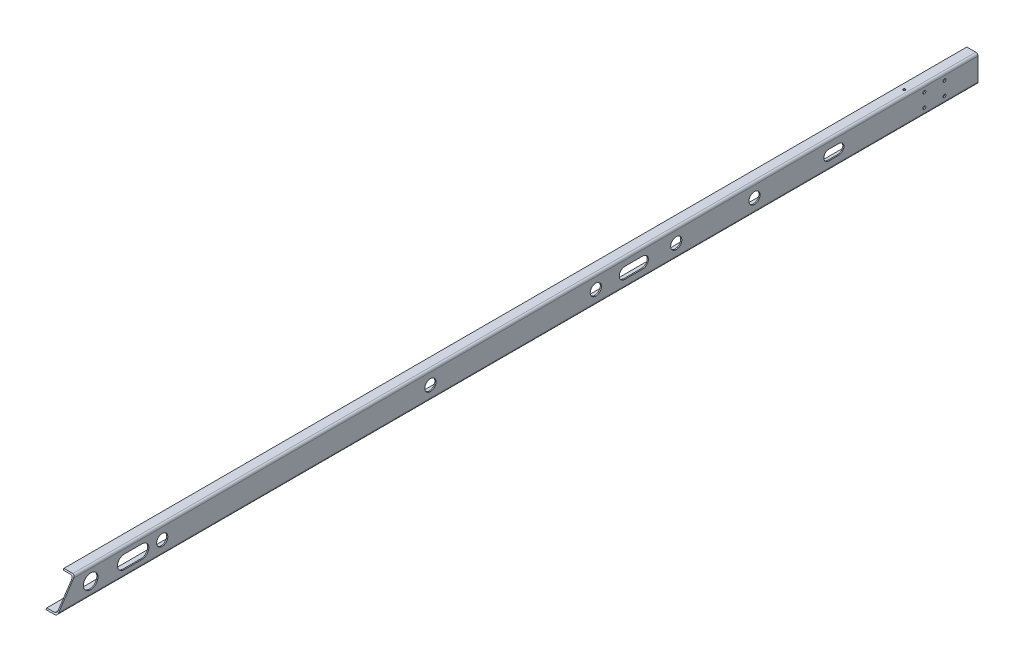
SolidWorks part; units mm, degrees
ref_plane "前视基准面" through (0, 0, 0) normal (0, 0, 1) x (1, 0, 0)
ref_plane "上视基准面" through (0, 0, 0) normal (0, 1, 0) x (1, 0, 0)
ref_plane "右视基准面" through (0, 0, 0) normal (1, 0, 0) x (0, 0, -1)
sketch "草图1" plane through (0, 0, 0) normal (0, 0, 1) x (1, 0, 0)
  line L24 (626.1756, -48.4289) -> (666.1756, -48.4289)
  line L25 (676.1756, -38.4289) -> (676.1756, 61.5711)
  line L26 (666.1756, 71.5711) -> (626.1756, 71.5711)
  line L27 (626.1756, 71.5711) -> (626.1756, 66.5711)
  line L28 (626.1756, 66.5711) -> (661.1756, 66.5711)
  line L29 (671.1756, 56.5711) -> (671.1756, -33.4289)
  line L30 (661.1756, -43.4289) -> (626.1756, -43.4289)
  line L31 (626.1756, -43.4289) -> (626.1756, -48.4289)
  arc A12 (666.1756, -48.4289) -> (676.1756, -38.4289) centre (666.1756, -38.4289) ccw
  arc A13 (676.1756, 61.5711) -> (666.1756, 71.5711) centre (666.1756, 61.5711) ccw
  arc A14 (671.1756, 56.5711) -> (661.1756, 66.5711) centre (661.1756, 56.5711) ccw
  arc A15 (661.1756, -43.4289) -> (671.1756, -33.4289) centre (661.1756, -33.4289) ccw
extrude "凸台-拉伸1" add sketch "草图1" along normal blind 4120
sketch "草图2" plane through (0, 71.5711, 0) normal (0, 1, 0) x (1, 0, 0)
  line L0 (626.1756, 0) -> (676.1756, 0)
  line L1 (651.1756, 0) -> (651.1756, -305)
  circle A0 centre (651.1756, -305) radius 5
extrude "切除-拉伸1" cut sketch "草图2" against normal blind 10
sketch "草图3" plane through (676.1756, 0, 0) normal (1, 0, 0) x (0, 0, -1)
  line L8 (-667.5, 34.0711) -> (-622.5, 34.0711)
  line L9 (-622.5, -10.9289) -> (-667.5, -10.9289)
  line L23 (-3820, 41.5711) -> (-3740, 41.5711)
  line L24 (-3740, -18.4289) -> (-3820, -18.4289)
  circle A0 centre (-225, 41.5711) radius 6.5
  circle A1 centre (-135, 41.5711) radius 6.5
  circle A2 centre (-135, -18.4289) radius 6.5
  circle A3 centre (-225, -18.4289) radius 6.5
  arc A4 (-622.5, -10.9289) -> (-622.5, 34.0711) centre (-622.5, 11.5711) ccw
  arc A5 (-667.5, 34.0711) -> (-667.5, -10.9289) centre (-667.5, 11.5711) ccw
  circle A6 centre (-1000, 11.5711) radius 25
  circle A7 centre (-1350, 11.5711) radius 25
  circle A8 centre (-3970, 11.5711) radius 22.5
  circle A9 centre (-3650, 11.5711) radius 25
  arc A10 (-3820, 41.5711) -> (-3820, -18.4289) centre (-3820, 11.5711) ccw
  arc A11 (-3740, -18.4289) -> (-3740, 41.5711) centre (-3740, 11.5711) ccw
  circle A12 centre (-1710, 11.5711) radius 25
  circle A13 centre (-2450, 11.5711) radius 25
extrude "切除-拉伸2" cut sketch "草图3" against normal blind 10
sketch "草图4" plane through (676.1756, 0, 0) normal (1, 0, 0) x (0, 0, -1)
  line L6 (-1580, 36.5711) -> (-1500, 36.5711)
  line L7 (-1500, -13.4289) -> (-1580, -13.4289)
  arc A1 (-1580, 36.5711) -> (-1580, -13.4289) centre (-1580, 11.5711) ccw
  arc A2 (-1500, -13.4289) -> (-1500, 36.5711) centre (-1500, 11.5711) ccw
extrude "切除-拉伸3" cut sketch "草图4" against normal blind 10
sketch "草图5" plane through (676.1756, 0, 0) normal (1, 0, 0) x (0, 0, -1)
  line L0 (0, 41.5711) -> (-150, 41.5711)
  line L1 (0, -38.4289) -> (0, 61.5711) construction
  circle A0 centre (-225, 41.5711) radius 6.5
  circle A1 centre (-135, 41.5711) radius 6.5
  circle A2 centre (-135, -18.4289) radius 6.5
  circle A3 centre (-225, -18.4289) radius 6.5
  circle A4 centre (-150, 41.5711) radius 6.5
  circle A5 centre (-150, -18.4289) radius 6.5
  circle A6 centre (-240, -18.4289) radius 6.5
  circle A7 centre (-240, 41.5711) radius 6.5
extrude "切除-拉伸4" cut sketch "草图5" against normal blind 10
sketch "草图6" plane through (676.1756, 0, 0) normal (1, 0, 0) x (0, 0, -1)
  line L0 (-232.8464, 52.7731) -> (-232.8464, -32.1971)
  line L1 (-232.8464, -32.1971) -> (-210.7303, -32.1971)
  line L2 (-210.7303, -32.1971) -> (-210.7303, 54.2818)
  line L3 (-210.7303, 54.2818) -> (-232.8464, 52.7731)
  line L4 (-141.9395, 56.0058) -> (-142.9127, -30.5685)
  line L5 (-142.9127, -30.5685) -> (-122.7718, -30.5685)
  line L6 (-122.7718, -30.5685) -> (-119.3101, -30.5685)
  line L7 (-119.3101, -30.5685) -> (-119.3101, 56.0058)
  line L8 (-119.3101, 56.0058) -> (-141.9395, 56.0058)
extrude "凸台-拉伸4" add sketch "草图6" against normal blind 5
sketch "草图7" plane through (676.1756, 0, 0) normal (1, 0, 0) x (0, 0, -1)
  line L0 (-3970, 34.0711) -> (-3970, 44.0711)
  circle A0 centre (-3970, 11.5711) radius 22.5 construction
  circle A1 centre (-3970, 11.5711) radius 32.5
extrude "切除-拉伸5" cut sketch "草图7" against normal blind 10
sketch "草图8" plane through (676.1756, 0, 0) normal (1, 0, 0) x (0, 0, -1)
  line L0 (-4120, 71.5711) -> (-4040, 71.5711)
  line L1 (-4040, 71.5711) -> (-4120, -48.4289)
  line L2 (-4120, -48.4289) -> (-4120, 71.5711)
extrude "切除-拉伸6" cut sketch "草图8" against normal blind 63
